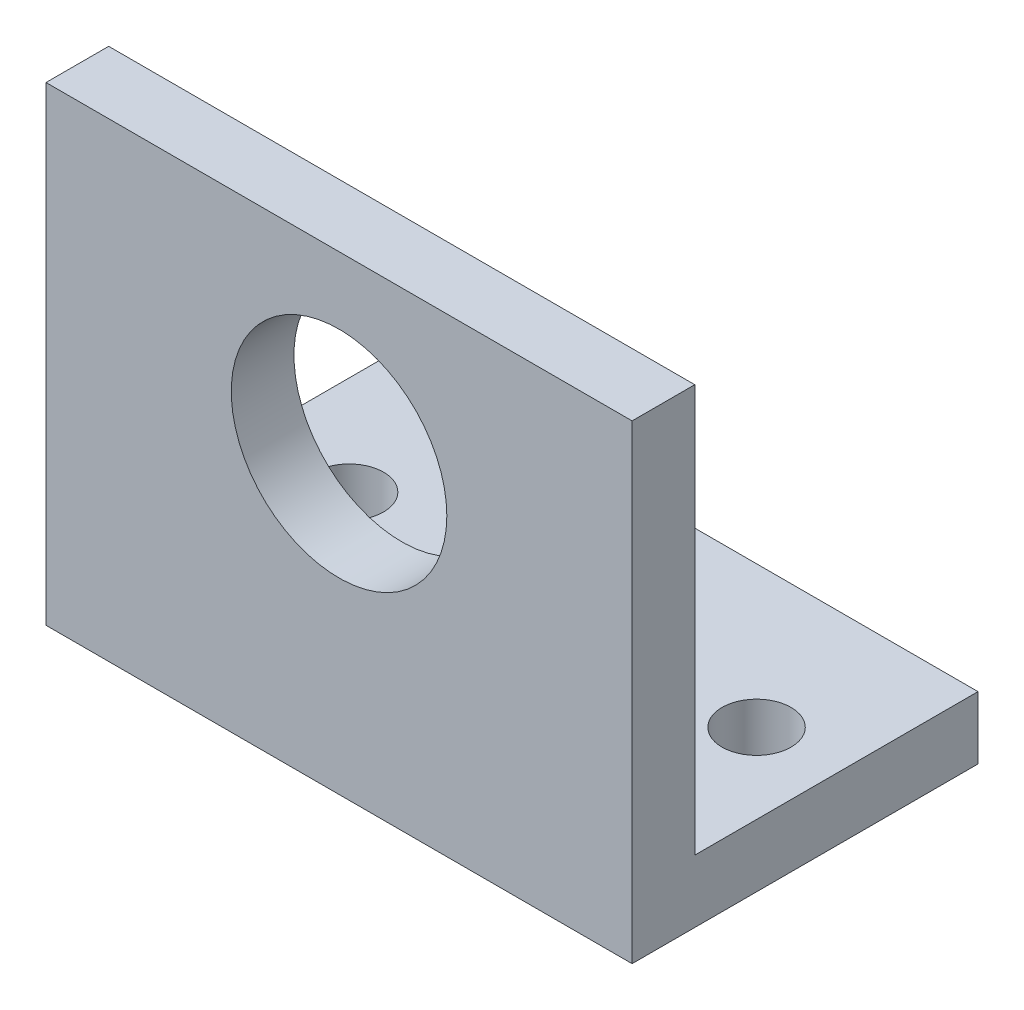
SolidWorks part; units mm, degrees
ref_plane "Front" through (0, 0, 0) normal (0, 0, 1) x (1, 0, 0)
ref_plane "Top" through (0, 0, 0) normal (0, 1, 0) x (1, 0, 0)
ref_plane "Right" through (0, 0, 0) normal (1, 0, 0) x (0, 0, -1)
sketch "Sketch1" plane through (0, 0, 0) normal (0, 1, 0) x (1, 0, 0)
  line L1 (-9.3507, -4.5187) -> (9.3507, -4.5187)
  line L2 (-9.3507, -4.5187) -> (-9.3507, 4.5187)
  line L3 (-9.3507, 4.5187) -> (9.3507, 4.5187)
  line L4 (9.3507, -4.5187) -> (9.3507, 4.5187)
  line L5 (-9.3507, -4.5187) -> (9.3507, 4.5187) construction
  line L6 (-9.3507, 4.5187) -> (9.3507, -4.5187) construction
  circle A0 centre (-6.1967, 0) radius 1.1
  circle A1 centre (6.8033, 0) radius 1.1
  point P0 (0, 0)
  dimension "D1" = 13
  dimension "D2" = 2.2
  dimension "D3" = 2.2
extrude "Boss-Extrude1" add sketch "Sketch1" along normal blind 2
sketch "Sketch2" plane through (0, 0, 4.5187) normal (0, 0, 1) x (1, 0, 0)
  line L0 (9.3507, 2) -> (9.3507, 0) construction
  line L1 (-9.3507, 0) -> (9.3507, 0)
  line L2 (-9.3507, 0) -> (-9.3507, 15)
  line L3 (-9.3507, 15) -> (9.3507, 15)
  line L4 (9.3507, 0) -> (9.3507, 15)
  circle A0 centre (0, 9.4213) radius 3.4392
  dimension "D1" = 0
  dimension "D2" = 15
extrude "Boss-Extrude2" add sketch "Sketch2" along normal blind 2
